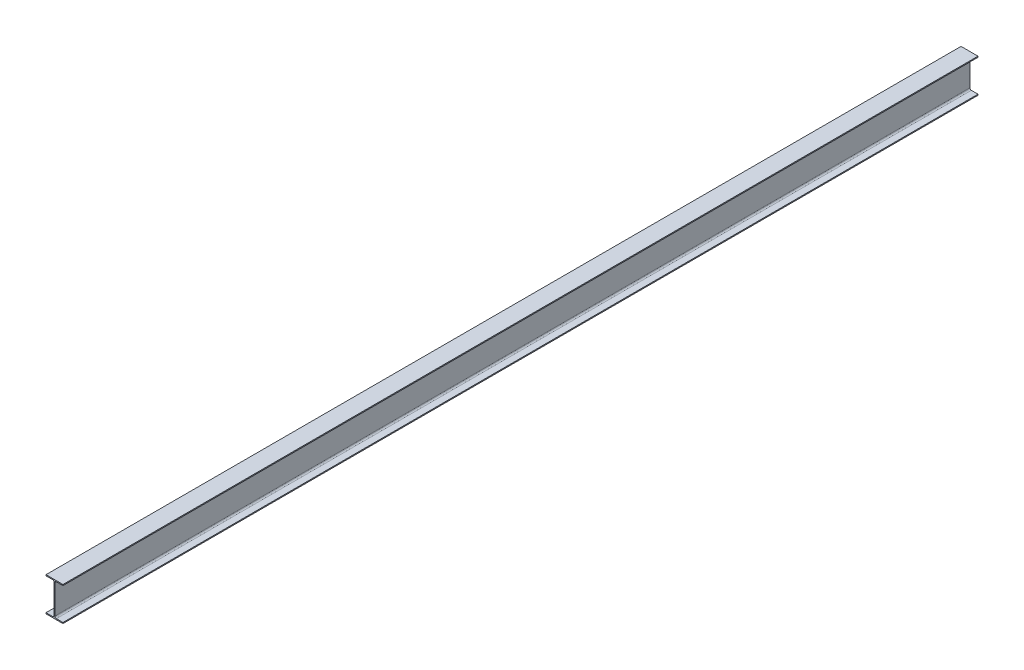
SolidWorks part; units mm, degrees
ref_plane "Front Plane" through (0, 0, 0) normal (0, 0, 1) x (1, 0, 0)
ref_plane "Top Plane" through (0, 0, 0) normal (0, 1, 0) x (1, 0, 0)
ref_plane "Right Plane" through (0, 0, 0) normal (1, 0, 0) x (0, 0, -1)
other "Configuration Table"
sketch "Sketch1" plane through (0, 0, 0) normal (0, 0, 1) x (1, 0, 0)
  line L0 (0, 0) -> (0, 300) construction
  line L1 (75, 0) -> (-75, 0)
  line L2 (-75, 0) -> (-75, 9)
  line L3 (-75, 9) -> (-16.25, 9)
  line L4 (3.25, 22) -> (3.25, 278)
  line L6 (-75, 291) -> (-75, 300)
  line L7 (-75, 300) -> (75, 300)
  line L8 (-3.25, 22) -> (-3.25, 278)
  line L9 (75, 291) -> (75, 300)
  line L10 (16.25, 291) -> (75, 291)
  line L11 (75, 9) -> (16.25, 9)
  line L12 (75, 0) -> (75, 9)
  line L13 (-16.25, 291) -> (-75, 291)
  arc A0 (16.25, 9) -> (3.25, 22) centre (16.25, 22) cw
  arc A1 (-3.25, 22) -> (-16.25, 9) centre (-16.25, 22) cw
  arc A2 (3.25, 278) -> (16.25, 291) centre (16.25, 278) cw
  arc A3 (-3.25, 278) -> (-16.25, 291) centre (-16.25, 278) ccw
  point P18 (3.25, 9)
  point P21 (-3.25, 9)
  point P24 (3.25, 291)
  point P27 (-3.25, 291)
  dimension "D6" = 13
  dimension "D1" = 300
  dimension "D2" = 150
  dimension "D3" = 6.5
  dimension "D4" = 9
  dimension "D5" = 9
extrude "Boss-Extrude1" add sketch "Sketch1" along normal blind 8090
